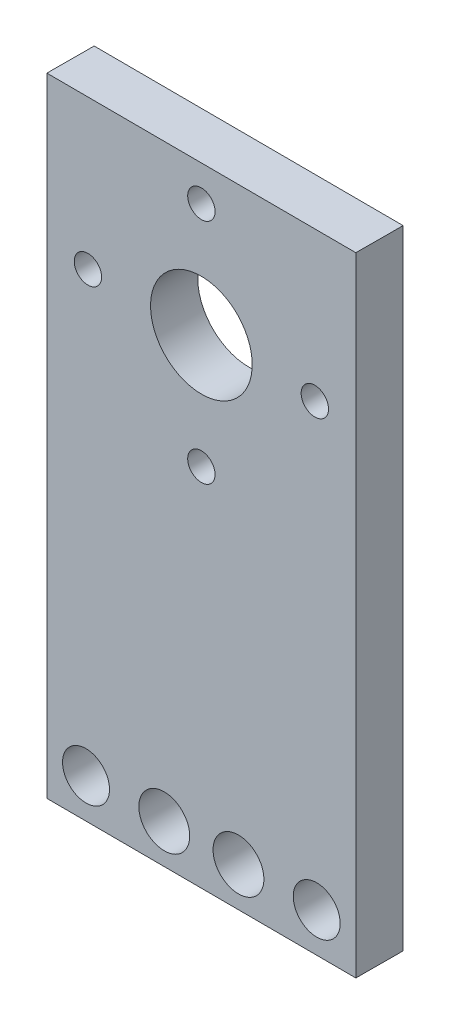
from build123d import *

# Parameters (mm, degrees)
SKETCH_2_W            = 39.483354071
SKETCH_2_H            = 80
EXTRUDE_1_DEPTH       = 6
SKETCH_3_R            = 3
CUT_EXTRUDE_1_DEPTH   = 10
HOLE_WIZARD_1_0_1_1_D = 6.5
SKETCH_6_R            = 6.5
CUT_EXTRUDE_2_DEPTH   = 218.242322412
HOLE_WIZARD_1_0_1_2_D = 3.5


with BuildPart() as part:
    # 草图2 → 凸台-拉伸1 (new body)
    with BuildSketch(Plane(origin=(0.031845394, 0, -9.289854674), x_dir=(0.9999941245437004, 0, 0.0034279553787324732), z_dir=(-0.0034279553787324732, 0, 0.9999941245437004))):
        with Locations((-185.77882216, 30.129161482)):
            Rectangle(SKETCH_2_W, SKETCH_2_H)
    extrude(amount=EXTRUDE_1_DEPTH)

    # 草图3 → 切除-拉伸1 (cut)
    with BuildSketch(Plane(origin=(0.011277662, 0, -3.289889926), x_dir=(0.9999941245437003, 0, 0.003427955378732479), z_dir=(-0.003427955378732479, 0, 0.9999941245437004))):
        with Locations((-200.520499196, -4.870838518)):
            Circle(SKETCH_3_R)
        with Locations((-171.037145125, -4.870838518)):
            Circle(SKETCH_3_R)
    extrude(amount=-CUT_EXTRUDE_1_DEPTH, mode=Mode.SUBTRACT)

    # Ø1.0 (1) 直径孔1 (through all)
    with Locations(Plane(origin=(0.011277662, 0, -3.289889926), x_dir=(0.9999941245437003, 0, 0.003427955378732479), z_dir=(-0.003427955378732479, 0, 0.9999941245437004))):
        with Locations((-190.520499196, -4.870838518), (-181.037145125, -4.870838518)):
            Hole(HOLE_WIZARD_1_0_1_1_D / 2)

    # 草图6 → 切除-拉伸2 (cut, through all)
    with BuildSketch(Plane(origin=(0.031845394, 0, -9.289854674), x_dir=(-0.9999941245437003, 0, -0.003427955378732479), z_dir=(0.003427955378732479, 0, -0.9999941245437004))):
        with Locations((185.777574302, 51.129161482)):
            Circle(SKETCH_6_R)
    extrude(amount=-CUT_EXTRUDE_2_DEPTH, mode=Mode.SUBTRACT)

    # Ø1.0 (1) 直径孔2 (through all)
    with Locations(Plane(origin=(0.011277662, 0, -3.289889926), x_dir=(0.9999941245437003, 0, 0.003427955378732479), z_dir=(-0.003427955378732479, 0, 0.9999941245437004))):
        with Locations((-185.777574302, 65.629161482), (-171.277574302, 51.129161482), (-185.777574302, 36.629161482), (-200.277574302, 51.129161482)):
            Hole(HOLE_WIZARD_1_0_1_2_D / 2)


solid = part.part
